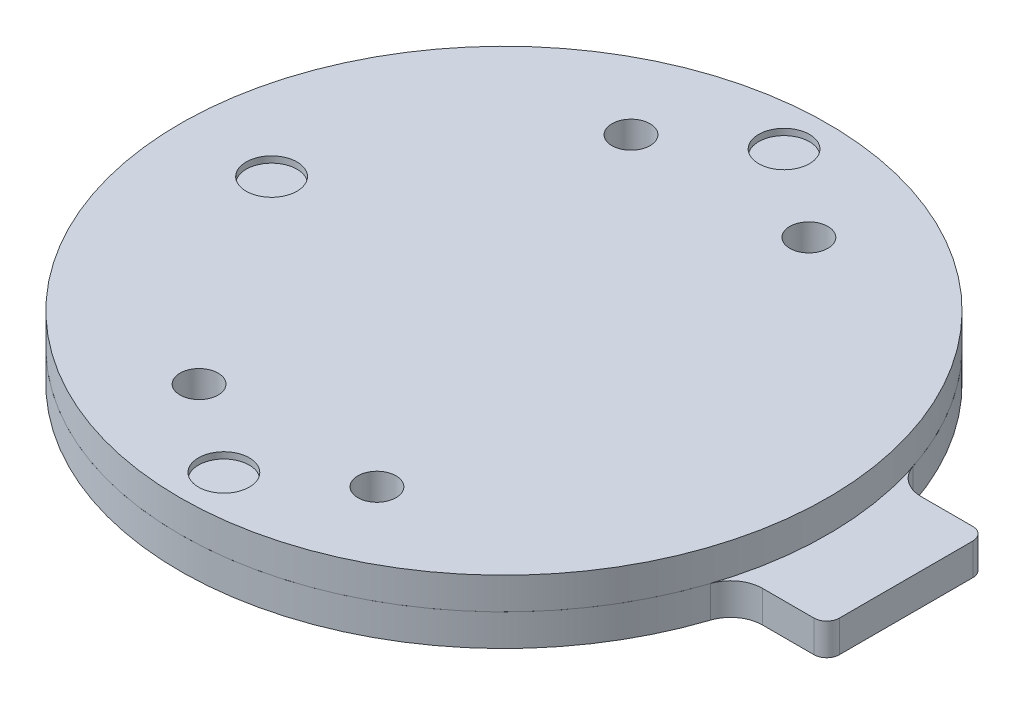
from build123d import *

# Parameters (mm, degrees)
SKETCH1_R           = 51
BOSS_EXTRUDE1_DEPTH = 5
BOSS_EXTRUDE2_DEPTH = 5
FILLET1_R           = 5
SKETCH4_R           = 51
BOSS_EXTRUDE3_DEPTH = 5
SKETCH5_R           = 3
CUT_EXTRUDE1_DEPTH  = 82.906804649
SKETCH6_R           = 4
CUT_EXTRUDE2_DEPTH  = 1


with BuildPart() as part:
    # Sketch1 → Boss-Extrude1 (new body)
    with BuildSketch(Plane(origin=(0, 0, 0), x_dir=(1, 0, 0), z_dir=(0, 1, 0))):
        with Locations(Location((0, 0, 0), (0, 0, 270))):
            Circle(SKETCH1_R)
    extrude(amount=BOSS_EXTRUDE1_DEPTH)

    # Sketch3 → Boss-Extrude2 (add)
    with BuildSketch(Plane(origin=(0, 5, 0), x_dir=(1, 0, 0), z_dir=(0, 1, 0))):
        with BuildLine():
            Line((49.444413233, 12.5), (61.306592452, 12.5))
            ThreePointArc((61.306592452, 12.5), (62.720806014, 11.914213562), (63.306592452, 10.5))
            Line((63.306592452, 10.5), (63.306592452, -10.5))
            ThreePointArc((63.306592452, -10.5), (62.720806014, -11.914213562), (61.306592452, -12.5))
            Line((61.306592452, -12.5), (49.444413233, -12.5))
            Line((49.444413233, -12.5), (49.444413233, 12.5))
        make_face()
    extrude(amount=-BOSS_EXTRUDE2_DEPTH)

    # Fillet1
    fillet1_edges = [part.edges().sort_by_distance(p)[0] for p in [
        (49.444413233, 2.5, 12.5),
        (49.444413233, 2.5, -12.5),
    ]]
    fillet(fillet1_edges, radius=FILLET1_R)


with BuildPart() as body_2:
    # Sketch4 → Boss-Extrude3 (new body)
    with BuildSketch(Plane(origin=(0, 5, 0), x_dir=(1, 0, 0), z_dir=(0, 1, 0))):
        with Locations(Location((0, 0, 0), (0, 0, 270))):
            Circle(SKETCH4_R)
    extrude(amount=BOSS_EXTRUDE3_DEPTH)


with BuildPart() as cut_extrude1_tool:
    # Sketch5 → Cut-Extrude1 (new, through all)
    with BuildSketch(Plane(origin=(0, 10, 0), x_dir=(1, 0, 0), z_dir=(0, 1, 0))):
        with Locations(Location((-14, 34, 0), (0, 0, 270))):
            Circle(SKETCH5_R)
        with Locations(Location((14, 34, 0), (0, 0, 270))):
            Circle(SKETCH5_R)
        with Locations(Location((14, -34, 0), (0, 0, 270))):
            Circle(SKETCH5_R)
        with Locations(Location((-14, -34, 0), (0, 0, 270))):
            Circle(SKETCH5_R)
    extrude(amount=-CUT_EXTRUDE1_DEPTH)


with BuildPart() as part_1:
    add(part.part)

    # Cut-Extrude1: cut by cut_extrude1_tool
    add(cut_extrude1_tool.part, mode=Mode.SUBTRACT)


with BuildPart() as body_2_1:
    add(body_2.part)

    # Cut-Extrude1: cut by cut_extrude1_tool
    add(cut_extrude1_tool.part, mode=Mode.SUBTRACT)

    # Sketch6 → Cut-Extrude2 (cut)
    with BuildSketch(Plane(origin=(0, 10, 0), x_dir=(1, 0, 0), z_dir=(0, 1, 0))):
        with Locations(Location((-36.58490914, 0, 0), (0, 0, 270))):
            Circle(SKETCH6_R)
        with Locations(Location((0, -44.09497379, 0), (0, 0, 270))):
            Circle(SKETCH6_R)
        with Locations(Location((0, 44.09497379, 0), (0, 0, 90))):
            Circle(SKETCH6_R)
    extrude(amount=-CUT_EXTRUDE2_DEPTH, mode=Mode.SUBTRACT)


solid = Compound([part_1.part, body_2_1.part])
